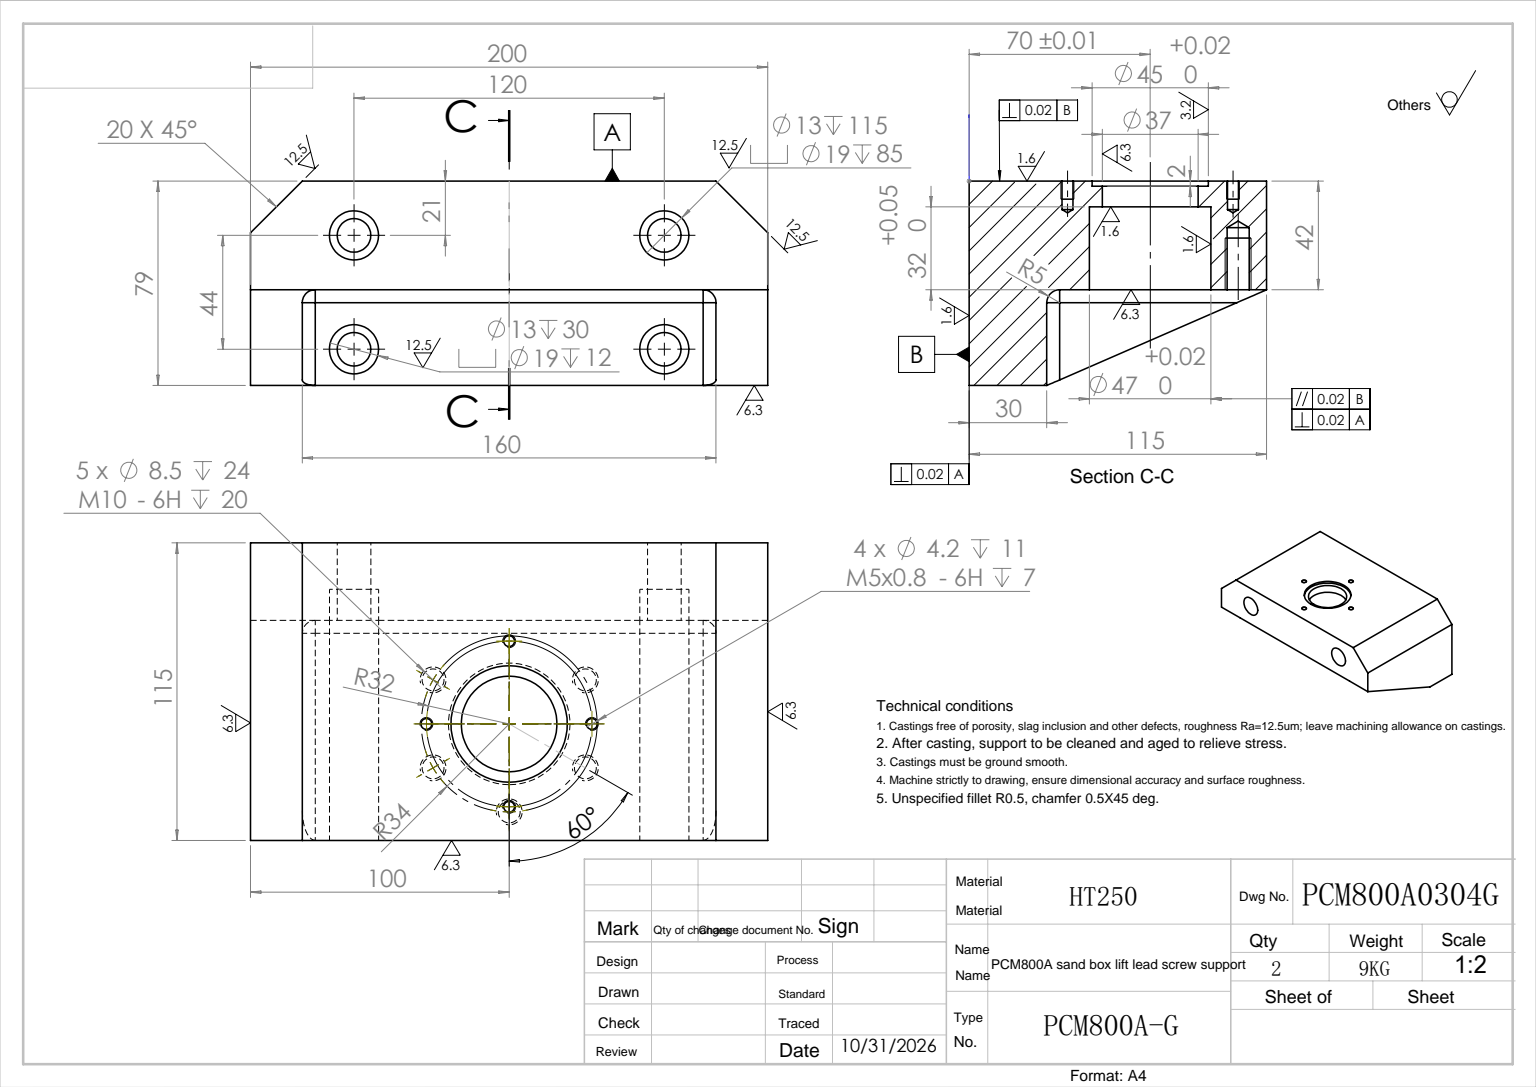
from build123d import *

# Parameters (mm, degrees)
EXTRUDE_1_DEPTH         = 115
SKETCH_2_W              = 200
SKETCH_2_H              = 37
EXTRUDE_2_DEPTH         = 30
EXTRUDE_3_DEPTH         = 20
SKETCH_4_R              = 22.5
CUT_EXTRUDE_1_DEPTH     = 2
SKETCH_5_R              = 18.5
CUT_EXTRUDE_2_DEPTH     = 8
CUT_EXTRUDE_3_REACH     = 169.29
SKETCH_6_R              = 23.5
SKETCH_7_R              = 9.5
CUT_EXTRUDE_4_DEPTH     = 85
SKETCH_8_R              = 6.5
CUT_EXTRUDE_5_DEPTH     = 154.186161255
SKETCH_9_R              = 2.5
CUT_EXTRUDE_6_DEPTH     = 10
FILLET_1_R              = 5
SKETCH_10_R             = 1
CUT_EXTRUDE_7_DEPTH     = 5
M5X0_8_1_D              = 4.2
M5X0_8_1_DEPTH          = 11
M5X0_8_1_TIP            = 1.2618073
HOLE_WIZARD_M10_1_D     = 8.5
HOLE_WIZARD_M10_1_DEPTH = 24
HOLE_WIZARD_M10_1_TIP   = 2.553657631
SKETCH_15_R             = 6.5
CUT_EXTRUDE_8_DEPTH     = 55
SKETCH_16_R             = 9.5
CUT_EXTRUDE_9_DEPTH     = 12


with BuildPart() as part:
    # 草图1 → 拉伸1 (new body)
    with BuildSketch(Plane.XY):
        Polygon((80, 0), (-80, 0), (-100, -20), (-100, -42), (100, -42), (100, -20), align=None)
    extrude(amount=EXTRUDE_1_DEPTH)

    # 草图2 → 拉伸2 (add)
    with BuildSketch(Plane.XY):
        with Locations((0, -60.5)):
            Rectangle(SKETCH_2_W, SKETCH_2_H)
    extrude(amount=EXTRUDE_2_DEPTH)

    # 草图3 → 拉伸3 (add)
    with BuildSketch(Plane.ZY.offset(100)):
        Polygon((115, -42), (30, -79), (30, -42), align=None)
    extrude_3 = extrude(amount=-EXTRUDE_3_DEPTH)

    # 镜向1: 拉伸3 across plane
    add(extrude_3.mirror(Plane(origin=(0, 0, 0), x_dir=(0, 0, 1), z_dir=(1, 0, 0))))

    # 草图4 → 切除-拉伸1 (cut)
    with BuildSketch(Plane(origin=(0, 0, 0), x_dir=(1, 0, 0), z_dir=(0, 1, 0))):
        with Locations(Location((0, -70, 0), (0, 0, 270))):
            Circle(SKETCH_4_R)
    extrude(amount=-CUT_EXTRUDE_1_DEPTH, mode=Mode.SUBTRACT)

    # 草图5 → 切除-拉伸2 (cut)
    with BuildSketch(Plane(origin=(0, -2, 0), x_dir=(1, 0, 0), z_dir=(0, 1, 0))):
        with Locations(Location((0, -70, 0), (0, 0, 270))):
            Circle(SKETCH_5_R)
    extrude(amount=-CUT_EXTRUDE_2_DEPTH, mode=Mode.SUBTRACT)

    # 草图6 → 切除-拉伸3 (cut, up to next)
    with BuildSketch(Plane(origin=(0, -10, 0), x_dir=(1, 0, 0), z_dir=(0, 1, 0)), mode=Mode.PRIVATE) as cut_extrude_3_sk1:
        with Locations(Location((0, -70, 0), (0, 0, 270))):
            Circle(SKETCH_6_R)
    cut_extrude_3_tool1 = extrude(cut_extrude_3_sk1.sketch, amount=-CUT_EXTRUDE_3_REACH, mode=Mode.PRIVATE) & part.part
    add(cut_extrude_3_tool1.solids().sort_by_distance((0, -10, 70))[0], mode=Mode.SUBTRACT)

    # 草图7 → 切除-拉伸4 (cut)
    with BuildSketch(Plane.XY.offset(115)):
        with Locations((60, -21)):
            Circle(SKETCH_7_R)
        with Locations((-60, -21)):
            Circle(SKETCH_7_R)
    extrude(amount=-CUT_EXTRUDE_4_DEPTH, mode=Mode.SUBTRACT)

    # 草图8 → 切除-拉伸5 (cut, through all)
    with BuildSketch(Plane.XY.offset(30)):
        with Locations((-60, -21)):
            Circle(SKETCH_8_R)
        with Locations((60, -21)):
            Circle(SKETCH_8_R)
    extrude(amount=-CUT_EXTRUDE_5_DEPTH, mode=Mode.SUBTRACT)

    # 草图9 → 切除-拉伸6 (cut)
    with BuildSketch(Plane.XZ.offset(42)):
        with Locations(Location((0, 104, 0), (0, 0, 270))):
            Circle(SKETCH_9_R)
        with Locations(Location((29.444863729, 87, 0), (0, 0, 270))):
            Circle(SKETCH_9_R)
        with Locations(Location((29.444863729, 53, 0), (0, 0, 270))):
            Circle(SKETCH_9_R)
        with Locations(Location((-29.444863729, 87, 0), (0, 0, 270))):
            Circle(SKETCH_9_R)
        with Locations(Location((-29.444863729, 53, 0), (0, 0, 270))):
            Circle(SKETCH_9_R)
    extrude(amount=-CUT_EXTRUDE_6_DEPTH, mode=Mode.SUBTRACT)

    # 圆角1
    fillet_1_edges = [part.edges().sort_by_distance(p)[0] for p in [
        (-80, -60.5, 30),
        (-80, -42, 72.5),
        (0, -42, 30),
        (80, -42, 72.5),
        (80, -60.5, 30),
    ]]
    fillet(fillet_1_edges, radius=FILLET_1_R)

    # 草图10 → 切除-拉伸7 (cut)
    with BuildSketch(Plane(origin=(0, 0, 0), x_dir=(1, 0, 0), z_dir=(0, 1, 0))):
        with Locations(Location((0, -38, 0), (0, 0, 270))):
            Circle(SKETCH_10_R)
        with Locations(Location((32, -70, 0), (0, 0, 270))):
            Circle(SKETCH_10_R)
        with Locations(Location((0, -102, 0), (0, 0, 270))):
            Circle(SKETCH_10_R)
        with Locations(Location((-32, -70, 0), (0, 0, 270))):
            Circle(SKETCH_10_R)
    extrude(amount=-CUT_EXTRUDE_7_DEPTH, mode=Mode.SUBTRACT)

    # M5x0.8 螺纹孔1
    with Locations(Plane(origin=(0, 0, 0), x_dir=(-1, 0, 0), z_dir=(0, 1, 0))):
        with Locations((0, 38), (-32, 70), (0, 102), (32, 70)):
            Hole(M5X0_8_1_D / 2, depth=M5X0_8_1_DEPTH)
            with Locations((0, 0, -(M5X0_8_1_DEPTH + M5X0_8_1_TIP / 2))):  # 118° drill point
                Cone(0, M5X0_8_1_D / 2, M5X0_8_1_TIP, mode=Mode.SUBTRACT)

    # M10 螺纹孔1
    with Locations(Plane.XZ.offset(42)):
        with Locations((29.444863729, 53), (29.444863729, 87), (0, 104), (-29.444863729, 87), (-29.444863729, 53)):
            Hole(HOLE_WIZARD_M10_1_D / 2, depth=HOLE_WIZARD_M10_1_DEPTH)
            with Locations((0, 0, -(HOLE_WIZARD_M10_1_DEPTH + HOLE_WIZARD_M10_1_TIP / 2))):  # 118° drill point
                Cone(0, HOLE_WIZARD_M10_1_D / 2, HOLE_WIZARD_M10_1_TIP, mode=Mode.SUBTRACT)

    # 草图15 → 切除-拉伸8 (cut)
    with BuildSketch(Plane.XY.offset(30)):
        with Locations((-60, -65)):
            Circle(SKETCH_15_R)
        with Locations((60, -65)):
            Circle(SKETCH_15_R)
    extrude(amount=-CUT_EXTRUDE_8_DEPTH, mode=Mode.SUBTRACT)

    # 草图16 → 切除-拉伸9 (cut)
    with BuildSketch(Plane.XY.offset(30)):
        with Locations((-60, -65)):
            Circle(SKETCH_16_R)
        with Locations((60, -65)):
            Circle(SKETCH_16_R)
    extrude(amount=-CUT_EXTRUDE_9_DEPTH, mode=Mode.SUBTRACT)


solid = part.part
